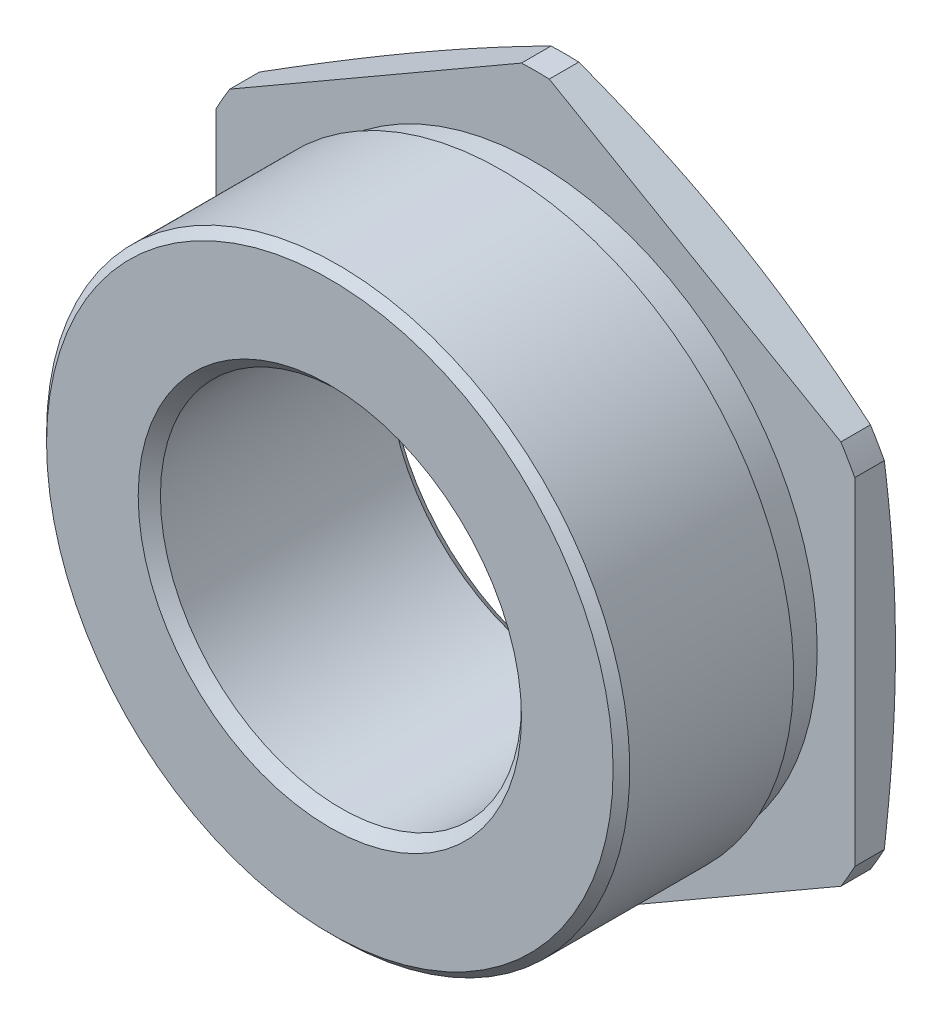
SolidWorks part; units mm, degrees
ref_plane "Front Plane" through (0, 0, 0) normal (0, 0, 1) x (1, 0, 0)
ref_plane "Top Plane" through (0, 0, 0) normal (0, 1, 0) x (1, 0, 0)
ref_plane "Right Plane" through (0, 0, 0) normal (1, 0, 0) x (0, 0, -1)
sketch "Sketch1" plane through (0, 0, 0) normal (0, 0, 1) x (1, 0, 0)
  line L1 (0, -66.3953) -> (57.5, -33.1976)
  line L2 (57.5, -33.1976) -> (57.5, 33.1976)
  line L3 (57.5, 33.1976) -> (0, 66.3953)
  line L4 (0, 66.3953) -> (-57.5, 33.1976)
  line L5 (-57.5, 33.1976) -> (-57.5, -33.1976)
  line L6 (-57.5, -33.1976) -> (0, -66.3953)
  circle A0 centre (0, 0) radius 65
  circle A1 centre (0, 0) radius 57.5 construction
  dimension "D1" = 130
  dimension "D2" = 115
extrude "Boss-Extrude1" add sketch "Sketch1" along normal blind 8 contours L2 A0 L3 L4 L5 L6 L1
sketch "Sketch2" plane through (0, 0, 0) normal (0, 0, -1) x (-1, 0, 0)
  circle A0 centre (0, 0) radius 52.5
  dimension "D1" = 105
extrude "Boss-Extrude2" add sketch "Sketch2" against normal blind 45
cosmetic thread "Cosmetic Thread1" parameters "D2"=57.505
sketch "Sketch3" plane through (0, 0, 8) normal (0, 0, 1) x (1, 0, 0)
  circle A0 centre (0, 0) radius 52.5 construction
  circle A1 centre (0, 0) radius 52.5
  circle A2 centre (0, 0) radius 50.75
  dimension "D1" = 101.5
extrude "Cut-Extrude1" cut sketch "Sketch3" along normal blind 6
sketch "Sketch4" plane through (0, 0, 45) normal (0, 0, 1) x (1, 0, 0)
  circle A0 centre (0, 0) radius 32.5
  dimension "D1" = 65
extrude "Cut-Extrude2" cut sketch "Sketch4" against normal through all
chamfer "Chamfer1" distance 2 angle 45 2 edges at (32.5, 0, 45) (32.5, 0, 0)
chamfer "Chamfer2" distance 1.5 angle 45 1 edges at (-52.5, 0, 45)
sketch "Sketch5" plane through (0, 0, 0) normal (0, 0, -1) x (-1, 0, 0)
  circle A0 centre (0, 0) radius 55
  dimension "D1" = 110
extrude "Cut-Extrude3" cut sketch "Sketch5" against normal through all draft 75 flip side to cut
